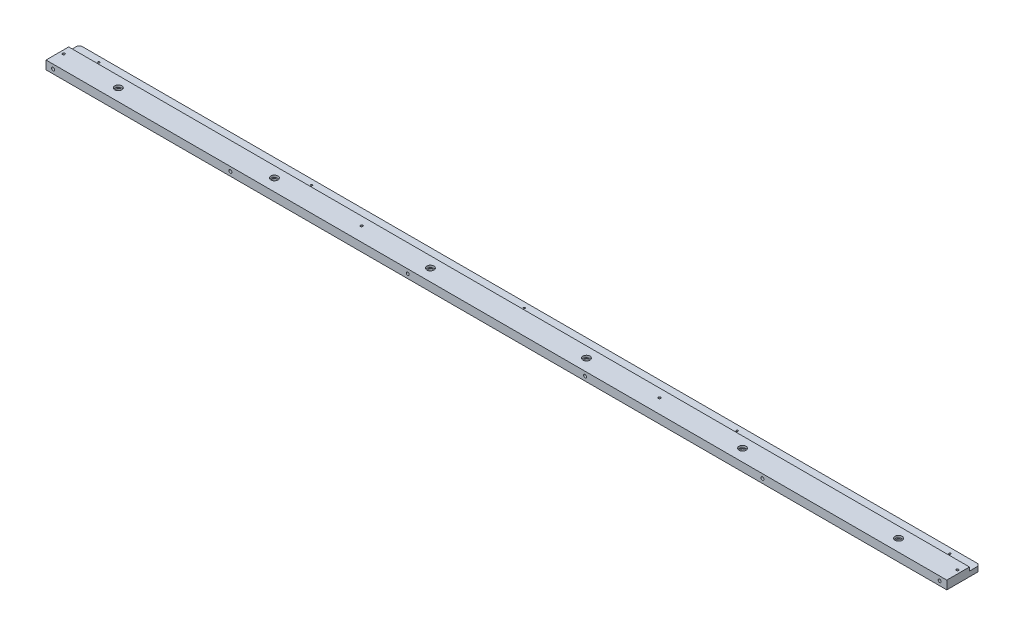
SolidWorks part; units mm, degrees
material "A6061"
ref_plane "前基準面" through (0, 0, 0) normal (0, 0, 1) x (1, 0, 0)
ref_plane "上基準面" through (0, 0, 0) normal (0, 1, 0) x (1, 0, 0)
ref_plane "右基準面" through (0, 0, 0) normal (1, 0, 0) x (0, 0, -1)
sketch "草图1" plane through (0, 0, 0) normal (0, 1, 0) x (1, 0, 0)
  line L1 (-635, -23.5) -> (635, -23.5)
  line L2 (-635, -23.5) -> (-635, 23.5)
  line L3 (-635, 23.5) -> (635, 23.5)
  line L4 (635, -23.5) -> (635, 23.5)
  line L5 (-635, -23.5) -> (635, 23.5) construction
  line L6 (-635, 23.5) -> (635, -23.5) construction
  point P0 (0, 0)
  dimension "D1" = 1270
  dimension "D2" = 47
extrude "凸台-拉伸1" add sketch "草图1" along normal mid plane 12
sketch "草图2" plane through (635, 0, 0) normal (1, 0, 0) x (0, 0, -1)
  line L1 (23.5, 6) -> (8.5, 6)
  line L2 (23.5, 6) -> (23.5, 1)
  line L3 (23.5, 1) -> (8.5, 1)
  line L4 (8.5, 6) -> (8.5, 1)
  dimension "D1" = 15
  dimension "D2" = 5
extrude "切除-拉伸1" cut sketch "草图2" against normal through all
chamfer "倒角1" distance 3 angle 45 2 edges at (-635, -2.5, -23.5) (635, -2.5, -23.5)
hole_wizard "M5 螺纹孔1" positions "草图3" profile "草图4" tap size "M5" standard "GB"
sketch "草图3" plane through (0, 0, 23.5) normal (0, 0, 1) x (1, 0, 0)
  line L0 (0, 0) -> (0, 147.4856) construction
  point P0 (-625, 0)
  point P6 (-375, 0)
  point P7 (-125, 0)
  point P8 (125, 0)
  point P9 (375, 0)
  point P10 (625, 0)
  dimension "D2" = 250
  dimension "D1" = 6
sketch "草图4" plane through (-625, 0, 23.5) normal (1, 0, 0) x (0, -1, 0)
  line L0 (0, 0) -> (0, 13.6618)
  line L1 (0, 13.6618) -> (2.1, 12.4)
  line L2 (2.1, 12.4) -> (2.1, 0)
  line L5 (2.1, 0) -> (0, 0)
  line L10 (0, 13.6618) -> (-2.1, 12.4) construction
  line L11 (0, -6.35) -> (0, 107.95) construction
  dimension "螺纹孔钻头直径" = 4.2
  dimension "螺纹孔钻头深度" = 12.4
  dimension "导头角度" = 118
cosmetic thread "孔螺蚊线1"
cosmetic thread "孔螺蚊线2"
cosmetic thread "孔螺蚊线3"
cosmetic thread "孔螺蚊线4"
cosmetic thread "孔螺蚊线5"
cosmetic thread "孔螺蚊线6"
hole_wizard "M4 螺纹孔1" positions "草图5" profile "草图6" tap size "M4" standard "GB" end condition through all
sketch "草图5" plane through (0, 6, 0) normal (0, 1, 0) x (1, 0, 0)
  line L0 (0, 0) -> (0, 95.1368) construction
  line L2 (635, -23.5) -> (635, 8.5) construction
  line L3 (-635, -23.5) -> (635, -23.5) construction
  point P0 (630, -3.5)
  point P7 (-630, -3.5)
  point P12 (210, -3.5)
  point P13 (-210, -3.5)
  dimension "D1" = 5
  dimension "D2" = 20
  dimension "D3" = 420
sketch "草图6" plane through (630, 6, 3.5) normal (1, 0, 0) x (0, 0, 1)
  line L0 (0, 0) -> (0, 12)
  line L1 (0, 12) -> (1.65, 12)
  line L2 (1.65, 12) -> (1.65, 0)
  line L5 (1.65, 0) -> (0, 0)
  line L11 (0, -6.35) -> (0, 107.95) construction
  dimension "通孔螺纹孔钻头直径" = 3.3
  dimension "通孔螺纹孔钻头深度" = 12
cosmetic thread "孔螺蚊线7"
cosmetic thread "孔螺蚊线8"
cosmetic thread "孔螺蚊线12"
cosmetic thread "孔螺蚊线13"
hole_wizard "M3 螺纹孔1" positions "草图8" profile "草图9" tap size "M3" standard "GB" end condition through all
sketch "草图8" plane through (0, -6, 0) normal (0, -1, 0) x (-1, 0, 0)
  line L0 (0, 8.5) -> (0, 23.5) construction
  line L1 (635, 8.5) -> (-635, 8.5) construction
  line L2 (632, 23.5) -> (-632, 23.5) construction
  point P0 (-600, 16)
  point P5 (-300, 16)
  point P6 (0, 16)
  point P7 (300, 16)
  point P8 (600, 16)
  dimension "D2" = 300
  dimension "D1" = 5
sketch "草图9" plane through (600, -6, -16) normal (1, 0, 0) x (0, 0, -1)
  line L0 (0, 0) -> (0, 12)
  line L1 (0, 12) -> (1.25, 12)
  line L2 (1.25, 12) -> (1.25, 0)
  line L5 (1.25, 0) -> (0, 0)
  line L11 (0, -6.35) -> (0, 107.95) construction
  dimension "通孔螺纹孔钻头直径" = 2.5
  dimension "通孔螺纹孔钻头深度" = 12
cosmetic thread "孔螺蚊线14"
cosmetic thread "孔螺蚊线15"
cosmetic thread "孔螺蚊线16"
cosmetic thread "孔螺蚊线17"
cosmetic thread "孔螺蚊线18"
hole_wizard "M8 螺纹孔1" positions "草图10" profile "草图11" tap size "M8" standard "ISO" end condition through all
sketch "草图10" plane through (0, -6, 0) normal (0, 1, 0) x (1, 0, 0)
  line L0 (0, 0) -> (0, -162.2294) construction
  line L2 (-635, -23.5) -> (635, -23.5) construction
  point P0 (550, -6.5)
  point P15 (330, -6.5)
  point P16 (110, -6.5)
  point P17 (-110, -6.5)
  point P18 (-330, -6.5)
  point P19 (-550, -6.5)
  dimension "D1" = 6
  dimension "D2" = 17
  dimension "D3" = 220
sketch "草图11" plane through (550, -6, 6.5) normal (1, 0, 0) x (0, 0, -1)
  line L0 (0, 0) -> (0, 12)
  line L1 (0, 12) -> (3.4, 12)
  line L2 (3.4, 12) -> (3.4, 0)
  line L5 (3.4, 0) -> (0, 0)
  line L11 (0, -6.35) -> (0, 107.95) construction
  dimension "通孔螺纹孔钻头直径" = 6.8
  dimension "通孔螺纹孔钻头深度" = 12
cosmetic thread "孔螺蚊线19"
cosmetic thread "孔螺蚊线20"
cosmetic thread "孔螺蚊线21"
cosmetic thread "孔螺蚊线22"
cosmetic thread "孔螺蚊线23"
cosmetic thread "孔螺蚊线24"
sketch "草图12" plane through (0, 6, 0) normal (0, 1, 0) x (1, 0, 0)
  circle A0 centre (550, -6.5) radius 5
  circle A1 centre (330, -6.5) radius 5
  circle A2 centre (110, -6.5) radius 5
  circle A3 centre (-110, -6.5) radius 5
  circle A4 centre (-330, -6.5) radius 5
  circle A5 centre (-550, -6.5) radius 5
  dimension "D1" = 10
  dimension "D2" = 6
extrude "切除-拉伸2" cut sketch "草图12" against normal blind 3
